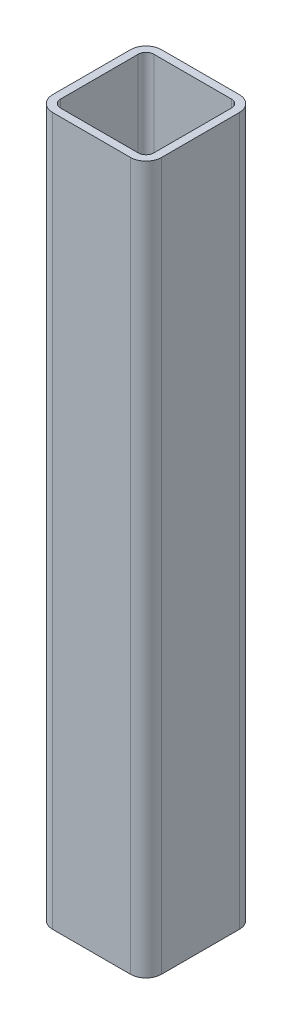
SolidWorks part; units mm, degrees
material "XRAAT"
ref_plane "前视基准面" through (0, 0, 0) normal (0, 0, 1) x (1, 0, 0)
ref_plane "上视基准面" through (0, 0, 0) normal (0, 1, 0) x (1, 0, 0)
ref_plane "右视基准面" through (0, 0, 0) normal (1, 0, 0) x (0, 0, -1)
sketch "草图1" plane through (0, 0, 0) normal (0, 0, 1) x (1, 0, 0)
  line L0 (0, 0) -> (0, 455)
  dimension "D1" = 455
other "结构用冷弯空心方钢(gb t6728-2002) 70×70×5(1)"
ref_plane "基准面1" through (0, 0, 0) normal (0, 1, 0) x (-1, 0, 0)
sketch "Sketch1" plane through (0, 0, 0) normal (0, 1, 0) x (-1, 0, 0)
  line L0 (-25, -30) -> (25, -30)
  line L1 (-30, -25) -> (-30, 25)
  line L2 (25, 30) -> (-25, 30)
  line L3 (30, 25) -> (30, -25)
  line L4 (-25, -35) -> (25, -35)
  line L5 (-35, -25) -> (-35, 25)
  line L6 (25, 35) -> (-25, 35)
  line L7 (35, 25) -> (35, -25)
  arc A0 (35, 25) -> (25, 35) centre (25, 25) ccw
  arc A1 (25, -35) -> (35, -25) centre (25, -25) ccw
  arc A2 (-35, -25) -> (-25, -35) centre (-25, -25) ccw
  arc A3 (-25, 35) -> (-35, 25) centre (-25, 25) ccw
  arc A4 (-25, 30) -> (-30, 25) centre (-25, 25) ccw
  arc A5 (30, 25) -> (25, 30) centre (25, 25) ccw
  arc A6 (25, -30) -> (30, -25) centre (25, -25) ccw
  arc A7 (-30, -25) -> (-25, -30) centre (-25, -25) ccw
  point P0 (-35, 0)
  point P1 (35, 0)
  point P2 (0, 35)
  point P3 (0, -35)
  point P4 (0, 0)
  point P5 (-35, -35)
  point P6 (35, -35)
  point P7 (35, 35)
  point P8 (-35, 35)
  point P33 (0, 0)
  dimension "D1" = 10
  dimension "D2" = 70
  dimension "D3" = 5
